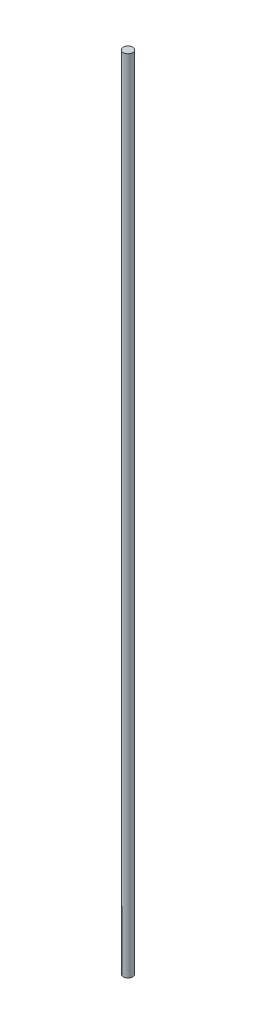
SolidWorks part; units mm, degrees
ref_plane "Front Plane" through (0, 0, 0) normal (0, 0, 1) x (1, 0, 0)
ref_plane "Top Plane" through (0, 0, 0) normal (0, 1, 0) x (1, 0, 0)
ref_plane "Right Plane" through (0, 0, 0) normal (1, 0, 0) x (0, 0, -1)
sketch "Sketch1" plane through (0, 0, 0) normal (0, 1, 0) x (1, 0, 0)
  circle A0 centre (0, 0) radius 2.5
  dimension "D1" = 5
extrude "Boss-Extrude1" add sketch "Sketch1" along normal blind 420
